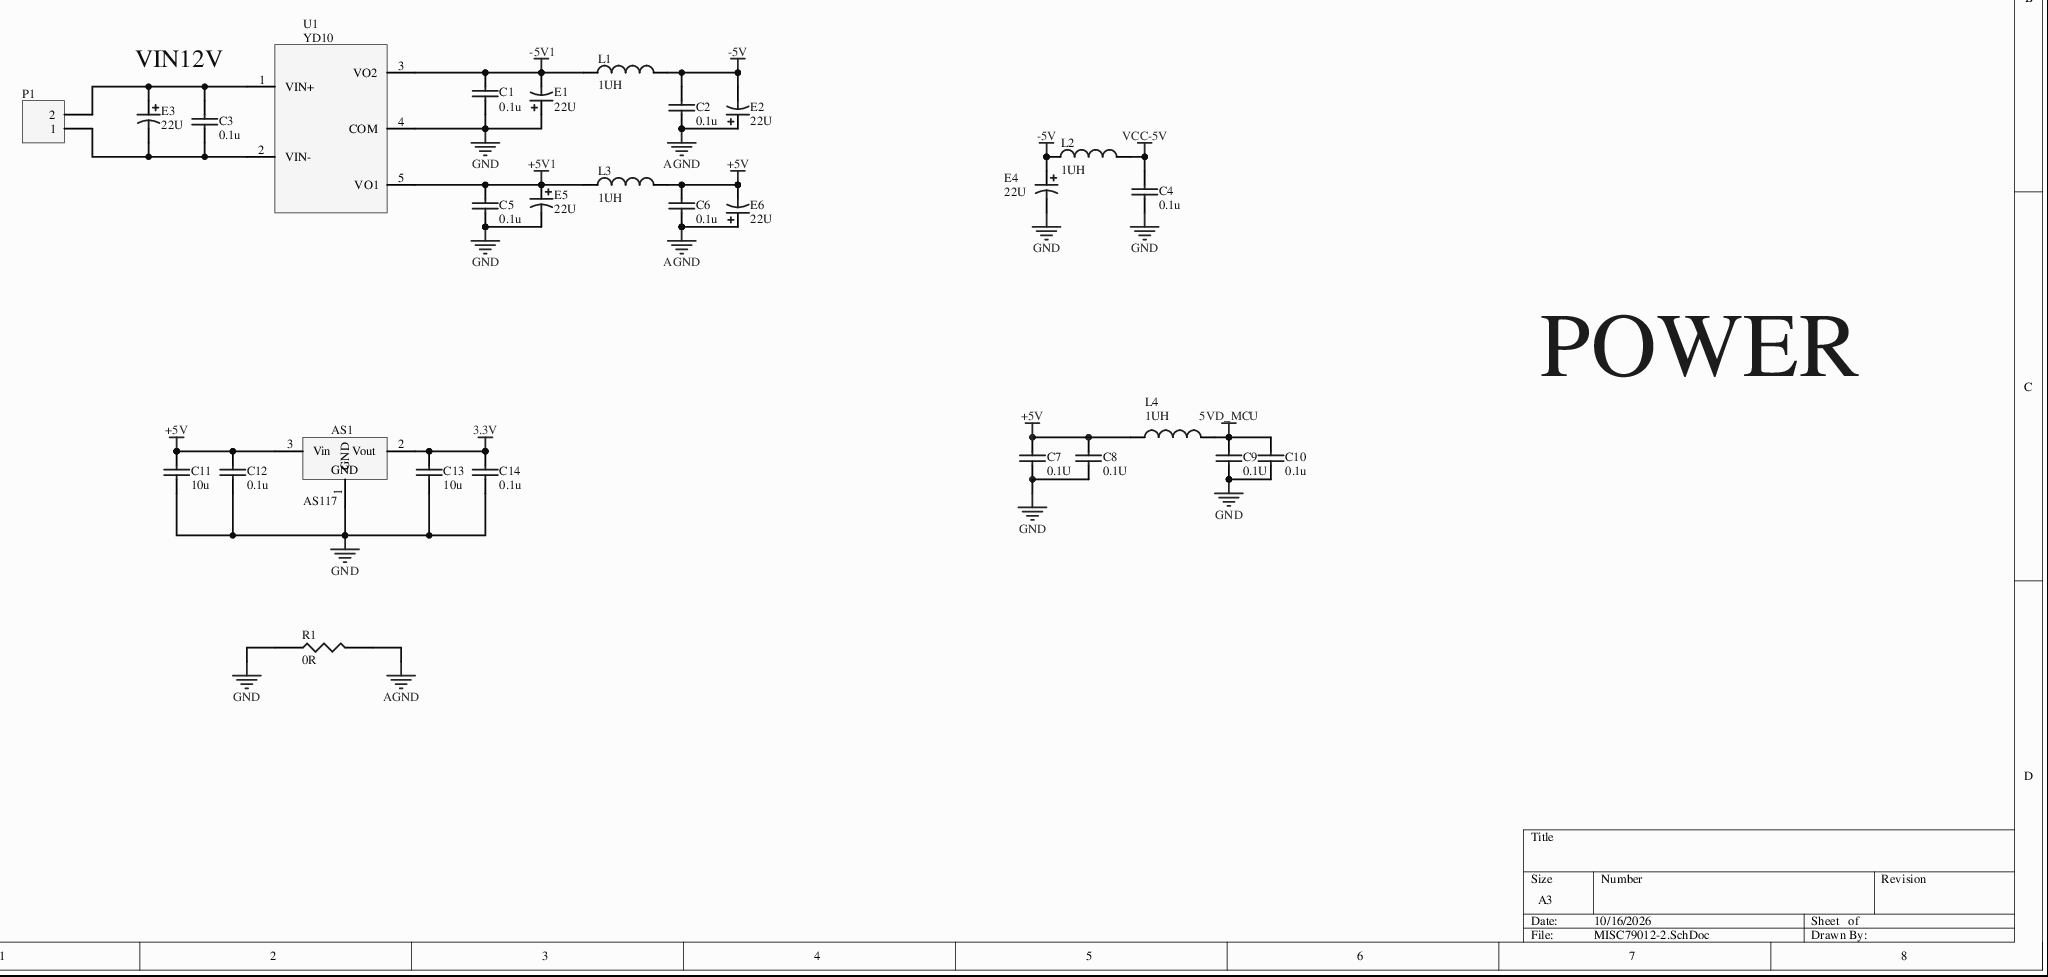
[diagram p0: MISC79012-2.SchDoc]
# Altium project MISC79012-4.PrjPcb
2 sheets, 54 parts. Net scope: global (net labels, ports and power ports of the same name join across sheets).
Board file: MISC79012.PcbDoc
Sheets:
  MISC79012-2.SchDoc
  MISC79012-3.SchDoc

## Sheet MISC79012-2.SchDoc
size A3; SheetNumber: 0; SheetTotal: 0

### Parts
AS1  AS117  [SOT223-4]
C1  0.1u  [0603]
C2  0.1u  [0603]
C3  0.1u  [0603]
C4  0.1u  [0603]
C5  0.1u  [0603]
C6  0.1u  [0603]
C7  0.1U  [0603]
C8  0.1U  [0603]
C9  0.1U  [0603]
C10  0.1u  [0603]
C11  10u  [1210]
C12  0.1u  [0603]
C13  10u  [1210]
C14  0.1u  [0603]
E1  22U  [1210]
E2  22U  [1210]
E3  22U  [1210]
E4  22U  [1210]
E5  22U  [1210]
E6  22U  [1210]
L1  1UH  [0805]
L2  1UH  [0805]
L3  1UH  [0805]
L4  1UH  [0805]
P1  (no value)  [MKDS3_2RMI]
R1  0R  [0603]
U1  YD10  [YD10]

### Nets
3.3V: AS1.2(Vout) C13.1 C14.1
5VD_MCU: C9.2 C10.1 L4.1
+5V: AS1.3(Vin) C6.1 C7.2 C8.2 C11.1 C12.1 E6.2 L3.2 L4.2
+5V1: C5.1 E5.1 L3.1 U1.5(VO1)
-5V: C2.1 E2.2 E4.1 L1.2 L2.1
-5V1: C1.1 E1.2 L1.1 U1.3(VO2)
AGND: C2.2 C6.2 E2.1 E6.1 R1.1
GND: AS1.1(GND) C1.2 C4.2 C5.2 C7.1 C8.1 C9.1 C10.2 C11.2 C12.2 C13.2 C14.2 E1.1 E4.2 E5.2 R1.2 U1.4(COM)
VCC-5V: C4.1 L2.2
NetC3_1: C3.1 E3.1 P1.2 U1.1(VIN+)
NetC3_2: C3.2 E3.2 P1.1 U1.2(VIN-)

### Notes on the sheet
- VIN12V
- POWER

### Library data of the parts
AS1 = Volt Reg: Voltage Regulator; Published: 24-Mar-1999; LatestRevisionDate: 17-Jul-2002; LatestRevisionNote: Re-released for DXP Platform.; PackageReference: D2PAK; Code_JEDEC: SMD-220; Publisher: Altium Limited
C1-C14 = CAP: Capacitor
E1-E6 = Cap Pol1: Polarized Capacitor (Radial); Published: 8-Jun-2000; LatestRevisionDate: 17-Jul-2002; LatestRevisionNote: Re-released for DXP Platform.; PackageReference: RB7.6-15; PackageDescription: Polarized Capacitor (Radial); 2 Leads; Value: 22U; Publisher: Altium Limited
L1-L4 = INDUCTOR: Text Field1: 10; Text Field2: 40
P1 = Header 2H: Header, 2-Pin, Right Angle; LatestRevisionDate: 17-Jul-2002; LatestRevisionNote: Re-released for DXP Platform.; Publisher: Altium Limited
R1 = RES1

## Sheet MISC79012-3.SchDoc
size A3; SheetNumber: 10; SheetTotal: 14
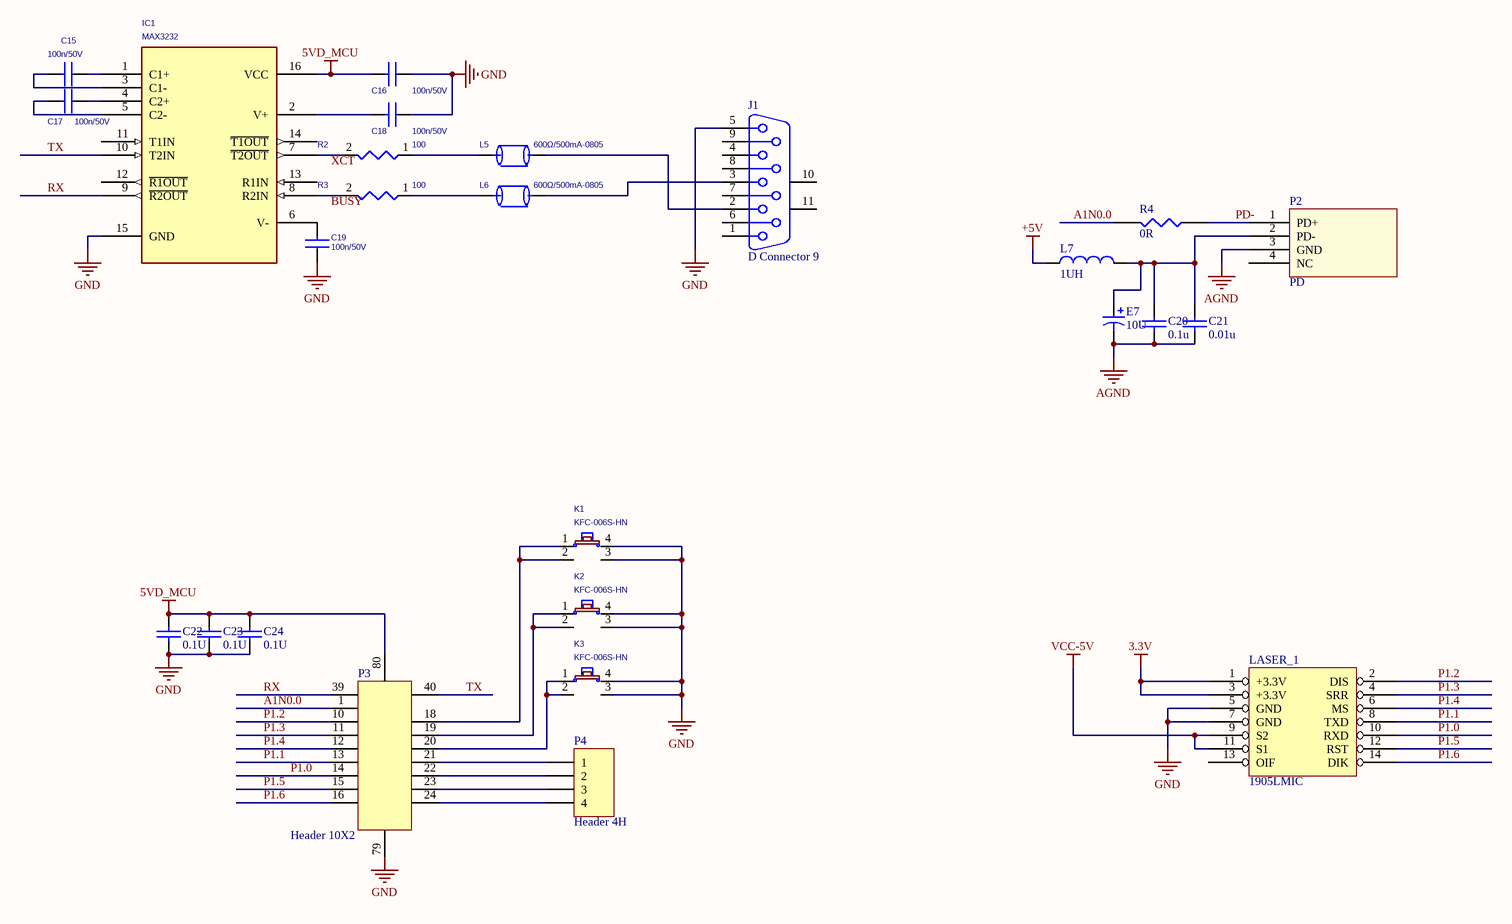
[diagram p1: MISC79012-3.SchDoc]

### Parts
C15  100n/50V  [0603]
C16  100n/50V  [0603]
C17  100n/50V  [0603]
C18  100n/50V  [0603]
C19  100n/50V  [0603]
C20  0.1u  [0603]
C21  0.01u  [0603]
C22  0.1U  [0603]
C23  0.1U  [0603]
C24  0.1U  [0603]
E7  10U  [1210]
IC1  MAX3232  [SOIC127P600-16N]
J1  D Connector 9  [DSUB1.385-2H9]
K1  KFC-006S-HN  [KNOB-SMD]
K2  KFC-006S-HN  [KNOB-SMD]
K3  KFC-006S-HN  [KNOB-SMD]
L5  600Ω/500mA-0805  [0805]
L6  600Ω/500mA-0805  [0805]
L7  1UH  [0805]
LASER_1  1905LMIC  [CLM-107-02-H-D-K-TR]
P2  PD  [guang2]
P3  Header 10X2  [c8051]
P4  Header 4H  [DIP-4]
R2  100  [0603]
R3  100  [0603]
R4  0R  [0603]

### Nets
3.3V: LASER_1.1(+3.3V) LASER_1.3(+3.3V)
5VD_MCU: C16.2 C22.2 C23.2 C24.2 IC1.16(VCC) P3.80
+5V: L7.1
AGND: C20.2 C21.2 E7.2 P2.3(GND)
GND: C16.1 C18.1 C19.1 C22.1 C23.1 C24.1 IC1.15(GND) J1.5 K1.3 K1.4 K2.3 K2.4 K3.3 K3.4 LASER_1.5(GND) LASER_1.7(GND) P3.79
VCC-5V: LASER_1.9(S2) LASER_1.11(S1)
A1N0.0: P3.1 R4.1
P1.0: LASER_1.10(RXD) P3.14
P1.1: LASER_1.8(TXD) P3.13
P1.2: LASER_1.2(DIS) P3.10
P1.3: LASER_1.4(SRR) P3.11
P1.4: LASER_1.6(MS) P3.12
P1.5: LASER_1.12(RST) P3.15
P1.6: LASER_1.14(DIK) P3.16
PD-: P2.1(PD+) R4.2
RX: IC1.9(~{R2OUT}) P3.39
TX: IC1.10(T2IN) P3.40
NetC15_1: C15.1 IC1.1(C1+)
NetC15_2: C15.2 IC1.3(C1-)
NetC17_1: C17.1 IC1.4(C2+)
NetC17_2: C17.2 IC1.5(C2-)
NetC18_2: C18.2 IC1.2(V+)
NetC19_2: C19.2 IC1.6(V-)
NetC20_1: C20.1 C21.1 E7.1 L7.2 P2.2(PD-)
NetIC1_7: IC1.7(~{T2OUT}) R2.2
NetIC1_8: IC1.8(R2IN) R3.2
NetJ1_2: J1.2 L5.2
NetJ1_3: J1.3 L6.2
NetK1_1: K1.1 K1.2 P3.18
NetK2_1: K2.1 K2.2 P3.19
NetK3_1: K3.1 K3.2 P3.20
NetL5_1: L5.1 R2.1
NetL6_1: L6.1 R3.1
NetP3_21: P3.21 P4.1
NetP3_22: P3.22 P4.2
NetP3_23: P3.23 P4.3
NetP3_24: P3.24 P4.4

Not connected (* = marked no-connect by the designer): IC1 11(T1IN) 12(~{R1OUT}) 13(R1IN) 14(~{T1OUT}); J1 1 4 6 7 8 9 10(MH1) 11(MH2); LASER_1 13(OIF); P2 4(NC)

### Notes on the sheet
- Labels drawn without touching a wire or pin: BUSY, XCT

### Library data of the parts
C15-C19 = CAPACITOR NON-POL
C20-C24 = CAP: Capacitor
E7 = Cap Pol1: Polarized Capacitor (Radial); Value: 22U; Published: 8-Jun-2000; LatestRevisionDate: 17-Jul-2002; LatestRevisionNote: Re-released for DXP Platform.; PackageReference: RB7.6-15; PackageDescription: Polarized Capacitor (Radial); 2 Leads; Publisher: Altium Limited
J1 = D Connector 9: Receptacle Assembly, 9 Position, Right Angle; PackageDocument: O; Positions: 9; Published: 15-Jun-2001; LatestRevisionDate: 17-Jul-2002; LatestRevisionNote: Re-released for DXP Platform.; DatasheetDocument: 1-Sep-1999; PackageReference: 788750; Orientation: Right Angle; Gender: Receptacle; Publisher: Altium Limited
K1-K3 = KNOB-SMD
L5 L6 = BEAD: Part Number: 20.43.10.0007.01; 替: 1; 厂: TDK; 规: TDK_MMZ2012S601AT000; Value1: 600Ω/500mA-0805; 物: 0805
L7 = INDUCTOR: Text Field1: 10; Text Field2: 40
LASER_1 = 1905LMI: Part Field 1: +5; Part Field 2: 0; Part Field 3: 0; Part Field 4: 0
P2 = FDDI
P3 = Header 10X2: Header, 10-Pin, Dual row; LatestRevisionDate: 17-Jul-2002; LatestRevisionNote: Re-released for DXP Platform.; Publisher: Altium Limited
P4 = Header 4H: Header, 4-Pin, Right Angle; LatestRevisionDate: 17-Jul-2002; LatestRevisionNote: Re-released for DXP Platform.; Publisher: Altium Limited
R2 R3 = SMDRXX_2: COMPHEIGHT: 0.000; MEMORY: NO; COMPGROUP: 0; COMPROT: 90; COMPLOC: [2325.000,2475.000]; COMPSIDE: TOP; DECOUPLER: NO; COMPKEY: NO; COMPLOCKED: NO; COMPFIXED: NO
R4 = RES1

## Nets that join several sheets
3.3V: MISC79012-2 (AS1.2 C13.1 C14.1), MISC79012-3 (LASER_1.1 LASER_1.3)
5VD_MCU: MISC79012-2 (C9.2 C10.1 L4.1), MISC79012-3 (6 pins)
+5V: MISC79012-2 (9 pins), MISC79012-3 (L7.1)
AGND: MISC79012-2 (5 pins), MISC79012-3 (C20.2 C21.2 E7.2 P2.3)
GND: MISC79012-2 (17 pins), MISC79012-3 (17 pins)
VCC-5V: MISC79012-2 (C4.1 L2.2), MISC79012-3 (LASER_1.9 LASER_1.11)